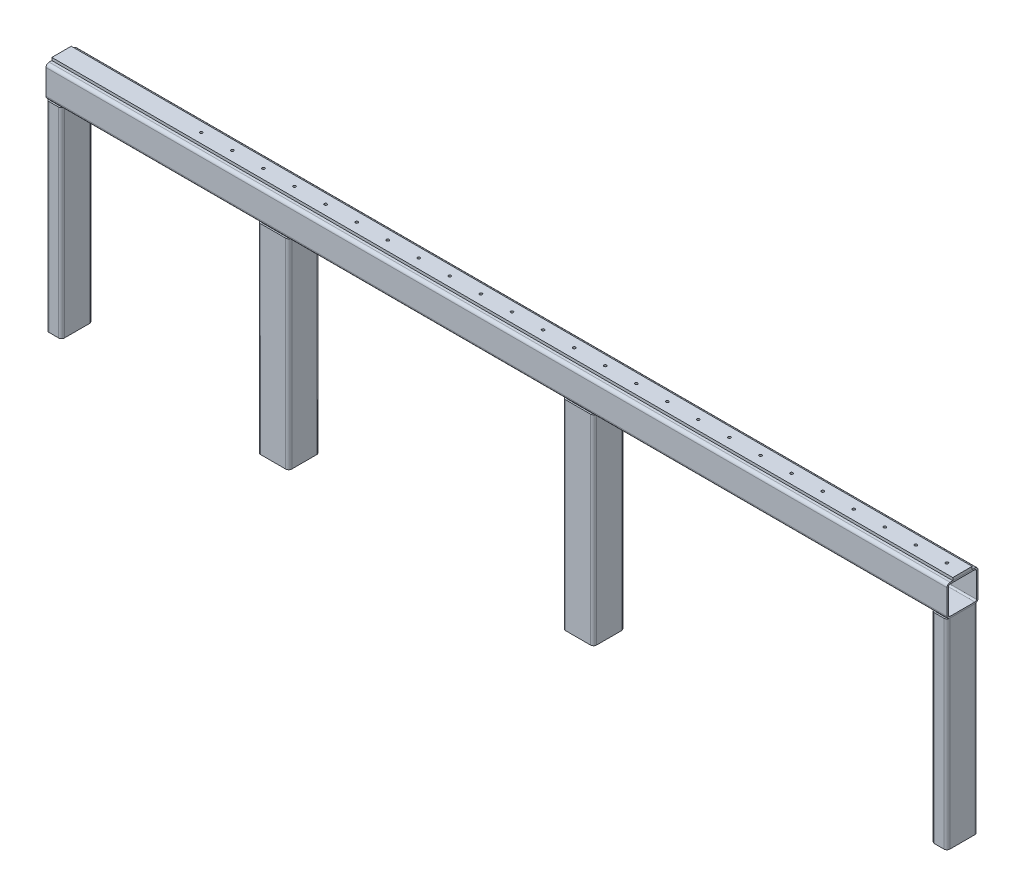
from build123d import *

# Parameters (mm, degrees)
GB_6728_1986_RECT_HOLLOW_SECTION_080_X_4_DEPTH = 515
GB_6728_1986_RECT_HOLLOW_SECTION_080_2_DEPTH   = 515
GB_6728_1986_SQUARE_HOLLOW_SECTION_080_X_DEPTH = 2280
BODY_START                                     = 226.27416998
BODY_3_RUN_ON_DEPTH                            = 246.27416998
BODY_START_2                                   = 2053.72583002
BODY_3_RUN_ON_2_DEPTH                          = 246.27416998
SKETCH2_W                                      = 2320
SKETCH2_H                                      = 50
BOSS_EXTRUDE1_DEPTH                            = 10
SKETCH4_W                                      = 2320
SKETCH4_H                                      = 50
CUT_EXTRUDE1_DEPTH                             = 3
LPATTERN1_COUNT                                = 25
LPATTERN1_PITCH                                = 80
SQUARE_TUBE_80_X_80_X_4_0_1_DEPTH              = 515
SQUARE_TUBE_80_X_80_X_4_0_1_2_DEPTH            = 515


with BuildPart() as part:
    # Sketch11 → GB/6728-1986 rect hollow section 080 X 40 X 4(1) (new body)
    with BuildSketch(Plane(origin=(0, 0, 0), x_dir=(-1, 0, 0), z_dir=(0, 1, 0))):
        with BuildLine():
            Line((-12, -40), (12, -40))
            ThreePointArc((12, -40), (17.656854249, -37.656854249), (20, -32))
            Line((20, -32), (20, 32))
            ThreePointArc((20, 32), (17.656854249, 37.656854249), (12, 40))
            Line((12, 40), (-12, 40))
            ThreePointArc((-12, 40), (-17.656854249, 37.656854249), (-20, 32))
            Line((-20, 32), (-20, -32))
            ThreePointArc((-20, -32), (-17.656854249, -37.656854249), (-12, -40))
        make_face()
        with BuildLine():
            Line((-12, -36), (12, -36))
            ThreePointArc((12, -36), (14.828427125, -34.828427125), (16, -32))
            Line((16, -32), (16, 32))
            ThreePointArc((16, 32), (14.828427125, 34.828427125), (12, 36))
            Line((12, 36), (-12, 36))
            ThreePointArc((-12, 36), (-14.828427125, 34.828427125), (-16, 32))
            Line((-16, 32), (-16, -32))
            ThreePointArc((-16, -32), (-14.828427125, -34.828427125), (-12, -36))
        make_face(mode=Mode.SUBTRACT)
    extrude(amount=GB_6728_1986_RECT_HOLLOW_SECTION_080_X_4_DEPTH)


with BuildPart() as body_2:
    # Sketch11 on segment 2 (carried to segment 2) → GB_6728-1986 rect hollow section 080 2 (new body)
    with BuildSketch(Plane(origin=(2280, 0, 0), x_dir=(-1, 0, 0), z_dir=(0, 1, 0))):
        with BuildLine():
            Line((-12, -40), (12, -40))
            ThreePointArc((12, -40), (17.656854249, -37.656854249), (20, -32))
            Line((20, -32), (20, 32))
            ThreePointArc((20, 32), (17.656854249, 37.656854249), (12, 40))
            Line((12, 40), (-12, 40))
            ThreePointArc((-12, 40), (-17.656854249, 37.656854249), (-20, 32))
            Line((-20, 32), (-20, -32))
            ThreePointArc((-20, -32), (-17.656854249, -37.656854249), (-12, -40))
        make_face()
        with BuildLine():
            Line((-12, -36), (12, -36))
            ThreePointArc((12, -36), (14.828427125, -34.828427125), (16, -32))
            Line((16, -32), (16, 32))
            ThreePointArc((16, 32), (14.828427125, 34.828427125), (12, 36))
            Line((12, 36), (-12, 36))
            ThreePointArc((-12, 36), (-14.828427125, 34.828427125), (-16, 32))
            Line((-16, 32), (-16, -32))
            ThreePointArc((-16, -32), (-14.828427125, -34.828427125), (-12, -36))
        make_face(mode=Mode.SUBTRACT)
    extrude(amount=GB_6728_1986_RECT_HOLLOW_SECTION_080_2_DEPTH)


with BuildPart() as body_3:
    # Sketch1 → GB/6728-1986 square hollow section 080 X 80 X 4(1) (new body)
    with BuildSketch(Plane(origin=(0, 555, 0), x_dir=(0, 1, 0), z_dir=(1, 0, 0))):
        with BuildLine():
            Line((-32, -40), (32, -40))
            ThreePointArc((32, -40), (37.656854249, -37.656854249), (40, -32))
            Line((40, -32), (40, 32))
            ThreePointArc((40, 32), (37.656854249, 37.656854249), (32, 40))
            Line((32, 40), (-32, 40))
            ThreePointArc((-32, 40), (-37.656854249, 37.656854249), (-40, 32))
            Line((-40, 32), (-40, -32))
            ThreePointArc((-40, -32), (-37.656854249, -37.656854249), (-32, -40))
        make_face()
        with BuildLine():
            Line((-32, -36), (32, -36))
            ThreePointArc((32, -36), (34.828427125, -34.828427125), (36, -32))
            Line((36, -32), (36, 32))
            ThreePointArc((36, 32), (34.828427125, 34.828427125), (32, 36))
            Line((32, 36), (-32, 36))
            ThreePointArc((-32, 36), (-34.828427125, 34.828427125), (-36, 32))
            Line((-36, 32), (-36, -32))
            ThreePointArc((-36, -32), (-34.828427125, -34.828427125), (-32, -36))
        make_face(mode=Mode.SUBTRACT)
    extrude(amount=GB_6728_1986_SQUARE_HOLLOW_SECTION_080_X_DEPTH)

    # body 3 cut square before the run-on
    split(bisect_by=Plane(origin=(226.27416998, 555, 0), x_dir=(0, 1, 0), z_dir=(1, 0, 0)), keep=Keep.TOP)

    # Sketch1 → body 3 run on (add)
    with BuildSketch(Plane(origin=(0, 555, 0), x_dir=(0, 1, 0), z_dir=(1, 0, 0)).offset(BODY_START)):
        with BuildLine():
            Line((-32, -40), (32, -40))
            ThreePointArc((32, -40), (37.656854249, -37.656854249), (40, -32))
            Line((40, -32), (40, 32))
            ThreePointArc((40, 32), (37.656854249, 37.656854249), (32, 40))
            Line((32, 40), (-32, 40))
            ThreePointArc((-32, 40), (-37.656854249, 37.656854249), (-40, 32))
            Line((-40, 32), (-40, -32))
            ThreePointArc((-40, -32), (-37.656854249, -37.656854249), (-32, -40))
        make_face()
        with BuildLine():
            Line((-32, -36), (32, -36))
            ThreePointArc((32, -36), (34.828427125, -34.828427125), (36, -32))
            Line((36, -32), (36, 32))
            ThreePointArc((36, 32), (34.828427125, 34.828427125), (32, 36))
            Line((32, 36), (-32, 36))
            ThreePointArc((-32, 36), (-34.828427125, 34.828427125), (-36, 32))
            Line((-36, 32), (-36, -32))
            ThreePointArc((-36, -32), (-34.828427125, -34.828427125), (-32, -36))
        make_face(mode=Mode.SUBTRACT)
    extrude(amount=-BODY_3_RUN_ON_DEPTH)

    # body 3 cut square before the run-on
    split(bisect_by=Plane(origin=(2053.72583002, 555, 0), x_dir=(0, -1, 0), z_dir=(-1, 0, 0)), keep=Keep.TOP)

    # Sketch1 → body 3 run on 2 (add)
    with BuildSketch(Plane(origin=(0, 555, 0), x_dir=(0, 1, 0), z_dir=(1, 0, 0)).offset(BODY_START_2)):
        with BuildLine():
            Line((-32, -40), (32, -40))
            ThreePointArc((32, -40), (37.656854249, -37.656854249), (40, -32))
            Line((40, -32), (40, 32))
            ThreePointArc((40, 32), (37.656854249, 37.656854249), (32, 40))
            Line((32, 40), (-32, 40))
            ThreePointArc((-32, 40), (-37.656854249, 37.656854249), (-40, 32))
            Line((-40, 32), (-40, -32))
            ThreePointArc((-40, -32), (-37.656854249, -37.656854249), (-32, -40))
        make_face()
        with BuildLine():
            Line((-32, -36), (32, -36))
            ThreePointArc((32, -36), (34.828427125, -34.828427125), (36, -32))
            Line((36, -32), (36, 32))
            ThreePointArc((36, 32), (34.828427125, 34.828427125), (32, 36))
            Line((32, 36), (-32, 36))
            ThreePointArc((-32, 36), (-34.828427125, 34.828427125), (-36, 32))
            Line((-36, 32), (-36, -32))
            ThreePointArc((-36, -32), (-34.828427125, -34.828427125), (-32, -36))
        make_face(mode=Mode.SUBTRACT)
    extrude(amount=BODY_3_RUN_ON_2_DEPTH)


with BuildPart() as body_4:
    # Sketch2 → Boss-Extrude1 (new body)
    with BuildSketch(Plane(origin=(0, 595, 0), x_dir=(1, 0, 0), z_dir=(0, 1, 0))):
        with Locations((1140, 0)):
            Rectangle(SKETCH2_W, SKETCH2_H)
    extrude(amount=BOSS_EXTRUDE1_DEPTH)

    # Sketch4 → Cut-Extrude1 (cut)
    with BuildSketch(Plane(origin=(0, 605, 0), x_dir=(1, 0, 0), z_dir=(0, 1, 0))):
        with Locations((1140, 0)):
            Rectangle(SKETCH4_W, SKETCH4_H)
    extrude(amount=-CUT_EXTRUDE1_DEPTH, mode=Mode.SUBTRACT)


with BuildPart() as m8_tapped_hole1_tool:
    # Sketch6 → M8 Tapped Hole1 (revolve)
    with BuildSketch(Plane(origin=(2260, 602, 0), x_dir=(0, 0, 1), z_dir=(1, 0, 0))):
        Polygon((0, 0), (0, 21.792926105), (3.4, 19.75), (3.4, 0), align=None)
    m8_tapped_hole1 = revolve(axis=Axis((2260, 608.35, 0), (0, -1, 0)))


with BuildPart() as body_3_1:
    add(body_3.part)

    # M8 Tapped Hole1: cut by m8_tapped_hole1_tool
    add(m8_tapped_hole1_tool.part, mode=Mode.SUBTRACT)


with BuildPart() as body_4_1:
    add(body_4.part)

    # M8 Tapped Hole1: cut by m8_tapped_hole1_tool
    add(m8_tapped_hole1_tool.part, mode=Mode.SUBTRACT)


with BuildPart() as lpattern1_tool:
    # LPattern1: M8 Tapped Hole1 ×25
    with Locations(*[(-i * LPATTERN1_PITCH, 0, 0) for i in range(1, LPATTERN1_COUNT)]):
        add(m8_tapped_hole1)


with BuildPart() as body_3_2:
    add(body_3_1.part)

    # LPattern1: cut by lpattern1_tool
    add(lpattern1_tool.part, mode=Mode.SUBTRACT)


with BuildPart() as body_4_2:
    add(body_4_1.part)

    # LPattern1: cut by lpattern1_tool
    add(lpattern1_tool.part, mode=Mode.SUBTRACT)


with BuildPart() as body_5:
    # Sketch12 → Square tube 80 X 80 X 4.0(1) (new body)
    with BuildSketch(Plane(origin=(565, 515, 0), x_dir=(1, 0, 0), z_dir=(0, -1, 0))):
        with BuildLine():
            Line((-32, -40), (32, -40))
            ThreePointArc((32, -40), (37.656854249, -37.656854249), (40, -32))
            Line((40, -32), (40, 32))
            ThreePointArc((40, 32), (37.656854249, 37.656854249), (32, 40))
            Line((32, 40), (-32, 40))
            ThreePointArc((-32, 40), (-37.656854249, 37.656854249), (-40, 32))
            Line((-40, 32), (-40, -32))
            ThreePointArc((-40, -32), (-37.656854249, -37.656854249), (-32, -40))
        make_face()
        with BuildLine():
            Line((-32, -36), (32, -36))
            ThreePointArc((32, -36), (34.828427125, -34.828427125), (36, -32))
            Line((36, -32), (36, 32))
            ThreePointArc((36, 32), (34.828427125, 34.828427125), (32, 36))
            Line((32, 36), (-32, 36))
            ThreePointArc((-32, 36), (-34.828427125, 34.828427125), (-36, 32))
            Line((-36, 32), (-36, -32))
            ThreePointArc((-36, -32), (-34.828427125, -34.828427125), (-32, -36))
        make_face(mode=Mode.SUBTRACT)
    extrude(amount=SQUARE_TUBE_80_X_80_X_4_0_1_DEPTH)


with BuildPart() as body_6:
    # Sketch12 on segment 2 (carried to segment 2) → Square tube 80 X 80 X 4.0_1 2 (new body)
    with BuildSketch(Plane(origin=(1350, 515, 0), x_dir=(1, 0, 0), z_dir=(0, -1, 0))):
        with BuildLine():
            Line((-32, -40), (32, -40))
            ThreePointArc((32, -40), (37.656854249, -37.656854249), (40, -32))
            Line((40, -32), (40, 32))
            ThreePointArc((40, 32), (37.656854249, 37.656854249), (32, 40))
            Line((32, 40), (-32, 40))
            ThreePointArc((-32, 40), (-37.656854249, 37.656854249), (-40, 32))
            Line((-40, 32), (-40, -32))
            ThreePointArc((-40, -32), (-37.656854249, -37.656854249), (-32, -40))
        make_face()
        with BuildLine():
            Line((-32, -36), (32, -36))
            ThreePointArc((32, -36), (34.828427125, -34.828427125), (36, -32))
            Line((36, -32), (36, 32))
            ThreePointArc((36, 32), (34.828427125, 34.828427125), (32, 36))
            Line((32, 36), (-32, 36))
            ThreePointArc((-32, 36), (-34.828427125, 34.828427125), (-36, 32))
            Line((-36, 32), (-36, -32))
            ThreePointArc((-36, -32), (-34.828427125, -34.828427125), (-32, -36))
        make_face(mode=Mode.SUBTRACT)
    extrude(amount=SQUARE_TUBE_80_X_80_X_4_0_1_2_DEPTH)


solid = Compound([part.part, body_2.part, body_3_2.part, body_4_2.part, body_5.part, body_6.part])
